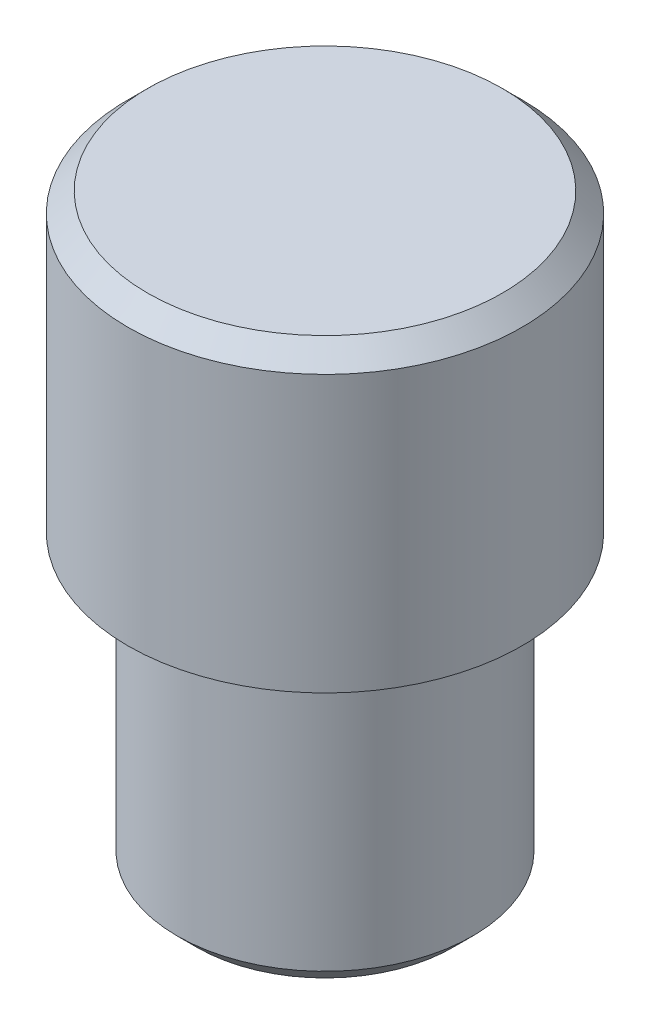
from build123d import *

# Parameters (mm, degrees)
SKETCH1_R           = 1.5
BOSS_EXTRUDE1_DEPTH = 3
SKETCH2_R           = 2
BOSS_EXTRUDE2_DEPTH = 3
CHAMFER1_SIZE       = 0.2


with BuildPart() as part:
    # Sketch1 → Boss-Extrude1 (new body)
    with BuildSketch(Plane(origin=(0, 0, 0), x_dir=(1, 0, 0), z_dir=(0, 1, 0))):
        with Locations(Location((0, 0, 0), (0, 0, 270))):
            Circle(SKETCH1_R)
    extrude(amount=BOSS_EXTRUDE1_DEPTH)

    # Sketch2 → Boss-Extrude2 (add)
    with BuildSketch(Plane(origin=(0, 3, 0), x_dir=(1, 0, 0), z_dir=(0, 1, 0))):
        with Locations(Location((0, 0, 0), (0, 0, 270))):
            Circle(SKETCH2_R)
    extrude(amount=BOSS_EXTRUDE2_DEPTH)

    # Chamfer1
    chamfer1_edges = [part.edges().sort_by_distance(p)[0] for p in [
        (0, 0, -1.5),
        (0, 6, -2),
    ]]
    chamfer(chamfer1_edges, length=CHAMFER1_SIZE)


solid = part.part
